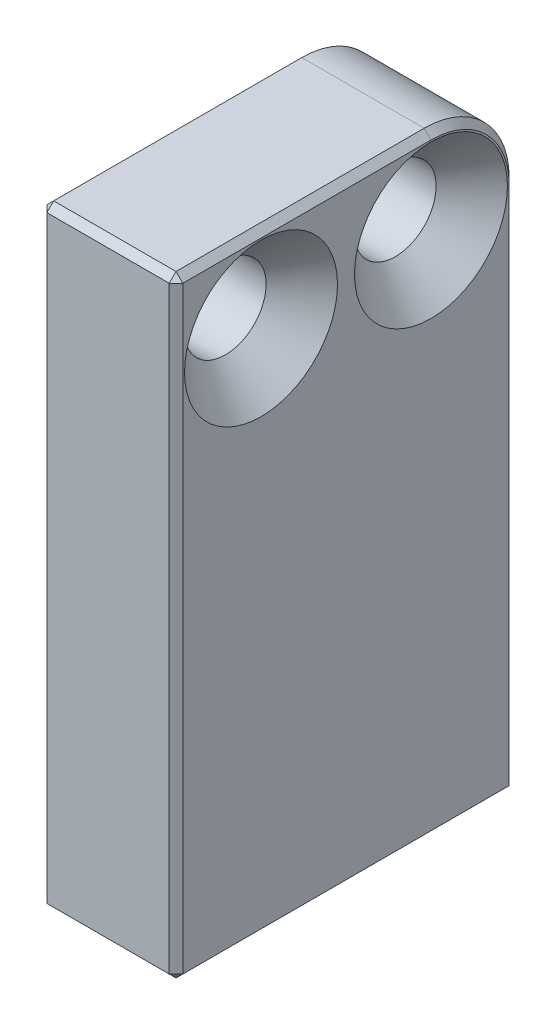
from build123d import *

# Parameters (mm, degrees)
SKETCH1_W                                            = 4
SKETCH1_H                                            = 10
BOSS_EXTRUDE1_DEPTH                                  = 18
HOLE_SIZE_SLOTTED_COUNTERSUNK_WOOD_SCREW_D           = 2.4
HOLE_SIZE_SLOTTED_COUNTERSUNK_WOOD_SCREW_CSINK_D     = 4.5
HOLE_SIZE_SLOTTED_COUNTERSUNK_WOOD_SCREW_CSINK_ANGLE = 90
M2_TAPPED_HOLE1_D                                    = 1.6
M2_TAPPED_HOLE1_DEPTH                                = 6.4
M2_TAPPED_HOLE1_TIP                                  = 0.480688495
FILLET1_R                                            = 2.5
CHAMFER1_SIZE                                        = 0.2


with BuildPart() as part:
    # Sketch1 → Boss-Extrude1 (new body)
    with BuildSketch(Plane(origin=(0, 0, 0), x_dir=(1, 0, 0), z_dir=(0, 1, 0))):
        with Locations((2, 5)):
            Rectangle(SKETCH1_W, SKETCH1_H)
    extrude(amount=BOSS_EXTRUDE1_DEPTH)

    # Hole size slotted countersunk wood screw type 1 (through all)
    with Locations(Plane(origin=(4, 0, 0), x_dir=(0, 0, -1), z_dir=(1, 0, 0))):
        with Locations((2.5, 15.5), (7.5, 15.5)):
            CounterSinkHole(HOLE_SIZE_SLOTTED_COUNTERSUNK_WOOD_SCREW_D / 2, HOLE_SIZE_SLOTTED_COUNTERSUNK_WOOD_SCREW_CSINK_D / 2, counter_sink_angle=HOLE_SIZE_SLOTTED_COUNTERSUNK_WOOD_SCREW_CSINK_ANGLE)

    # M2 Tapped Hole1
    with Locations(Plane(origin=(0, 0, 0), x_dir=(-1, 0, 0), z_dir=(0, -1, 0))):
        with Locations((-2, 2.5), (-2, 7.5)):
            Hole(M2_TAPPED_HOLE1_D / 2, depth=M2_TAPPED_HOLE1_DEPTH)
            with Locations((0, 0, -(M2_TAPPED_HOLE1_DEPTH + M2_TAPPED_HOLE1_TIP / 2))):  # 118° drill point
                Cone(0, M2_TAPPED_HOLE1_D / 2, M2_TAPPED_HOLE1_TIP, mode=Mode.SUBTRACT)

    # Fillet1
    fillet1_edges = [part.edges().sort_by_distance(p)[0] for p in [
        (2, 18, -10),
    ]]
    fillet(fillet1_edges, radius=FILLET1_R)

    # Chamfer1
    chamfer1_edges = [part.edges().sort_by_distance(p)[0] for p in [
        (4, 18, -3.75),
        (0, 15.5, -8.7),
        (0, 15.5, -3.7),
        (1.2, 0, -7.5),
        (1.2, 0, -2.5),
        (0, 18, -3.75),
        (0, 7.75, -10),
        (0, 17.267766953, -9.267766953),
        (4, 7.75, -10),
        (4, 17.267766953, -9.267766953),
        (2, 0, -10),
        (4, 0, -5),
        (2, 0, 0),
        (0, 0, -5),
        (4, 9, 0),
        (0, 9, 0),
        (2, 18, 0),
    ]]
    chamfer(chamfer1_edges, length=CHAMFER1_SIZE)


solid = part.part
